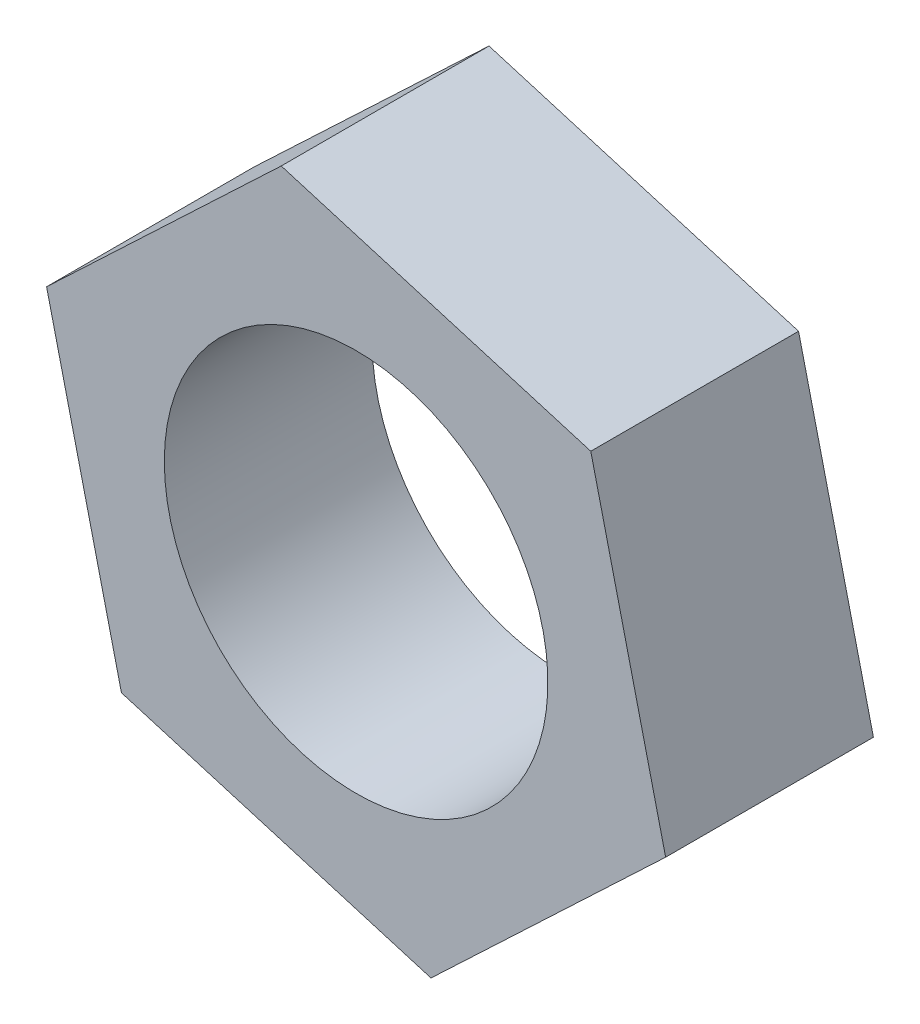
SolidWorks part; units mm, degrees
material "45"
ref_plane "Front Plane" through (0, 0, 0) normal (0, 0, 1) x (1, 0, 0)
ref_plane "Top Plane" through (0, 0, 0) normal (0, 1, 0) x (1, 0, 0)
ref_plane "Right Plane" through (0, 0, 0) normal (1, 0, 0) x (0, 0, -1)
sketch "Sketch1" plane through (0, 0, 0) normal (0, 0, 1) x (1, 0, 0)
  line L1 (38.7305, -11.5447) -> (29.3632, 27.7693)
  line L2 (29.3632, 27.7693) -> (-9.3673, 39.314)
  line L3 (-9.3673, 39.314) -> (-38.7305, 11.5447)
  line L4 (-38.7305, 11.5447) -> (-29.3632, -27.7693)
  line L5 (-29.3632, -27.7693) -> (9.3673, -39.314)
  line L6 (9.3673, -39.314) -> (38.7305, -11.5447)
  circle A0 centre (0, 0) radius 35 construction
  circle A1 centre (0, 0) radius 24
  dimension "D2" = 48
  dimension "D1" = 70
extrude "Boss-Extrude1" add sketch "Sketch1" along normal blind 26
cosmetic thread "Cosmetic Thread1" parameters "D2"=68
